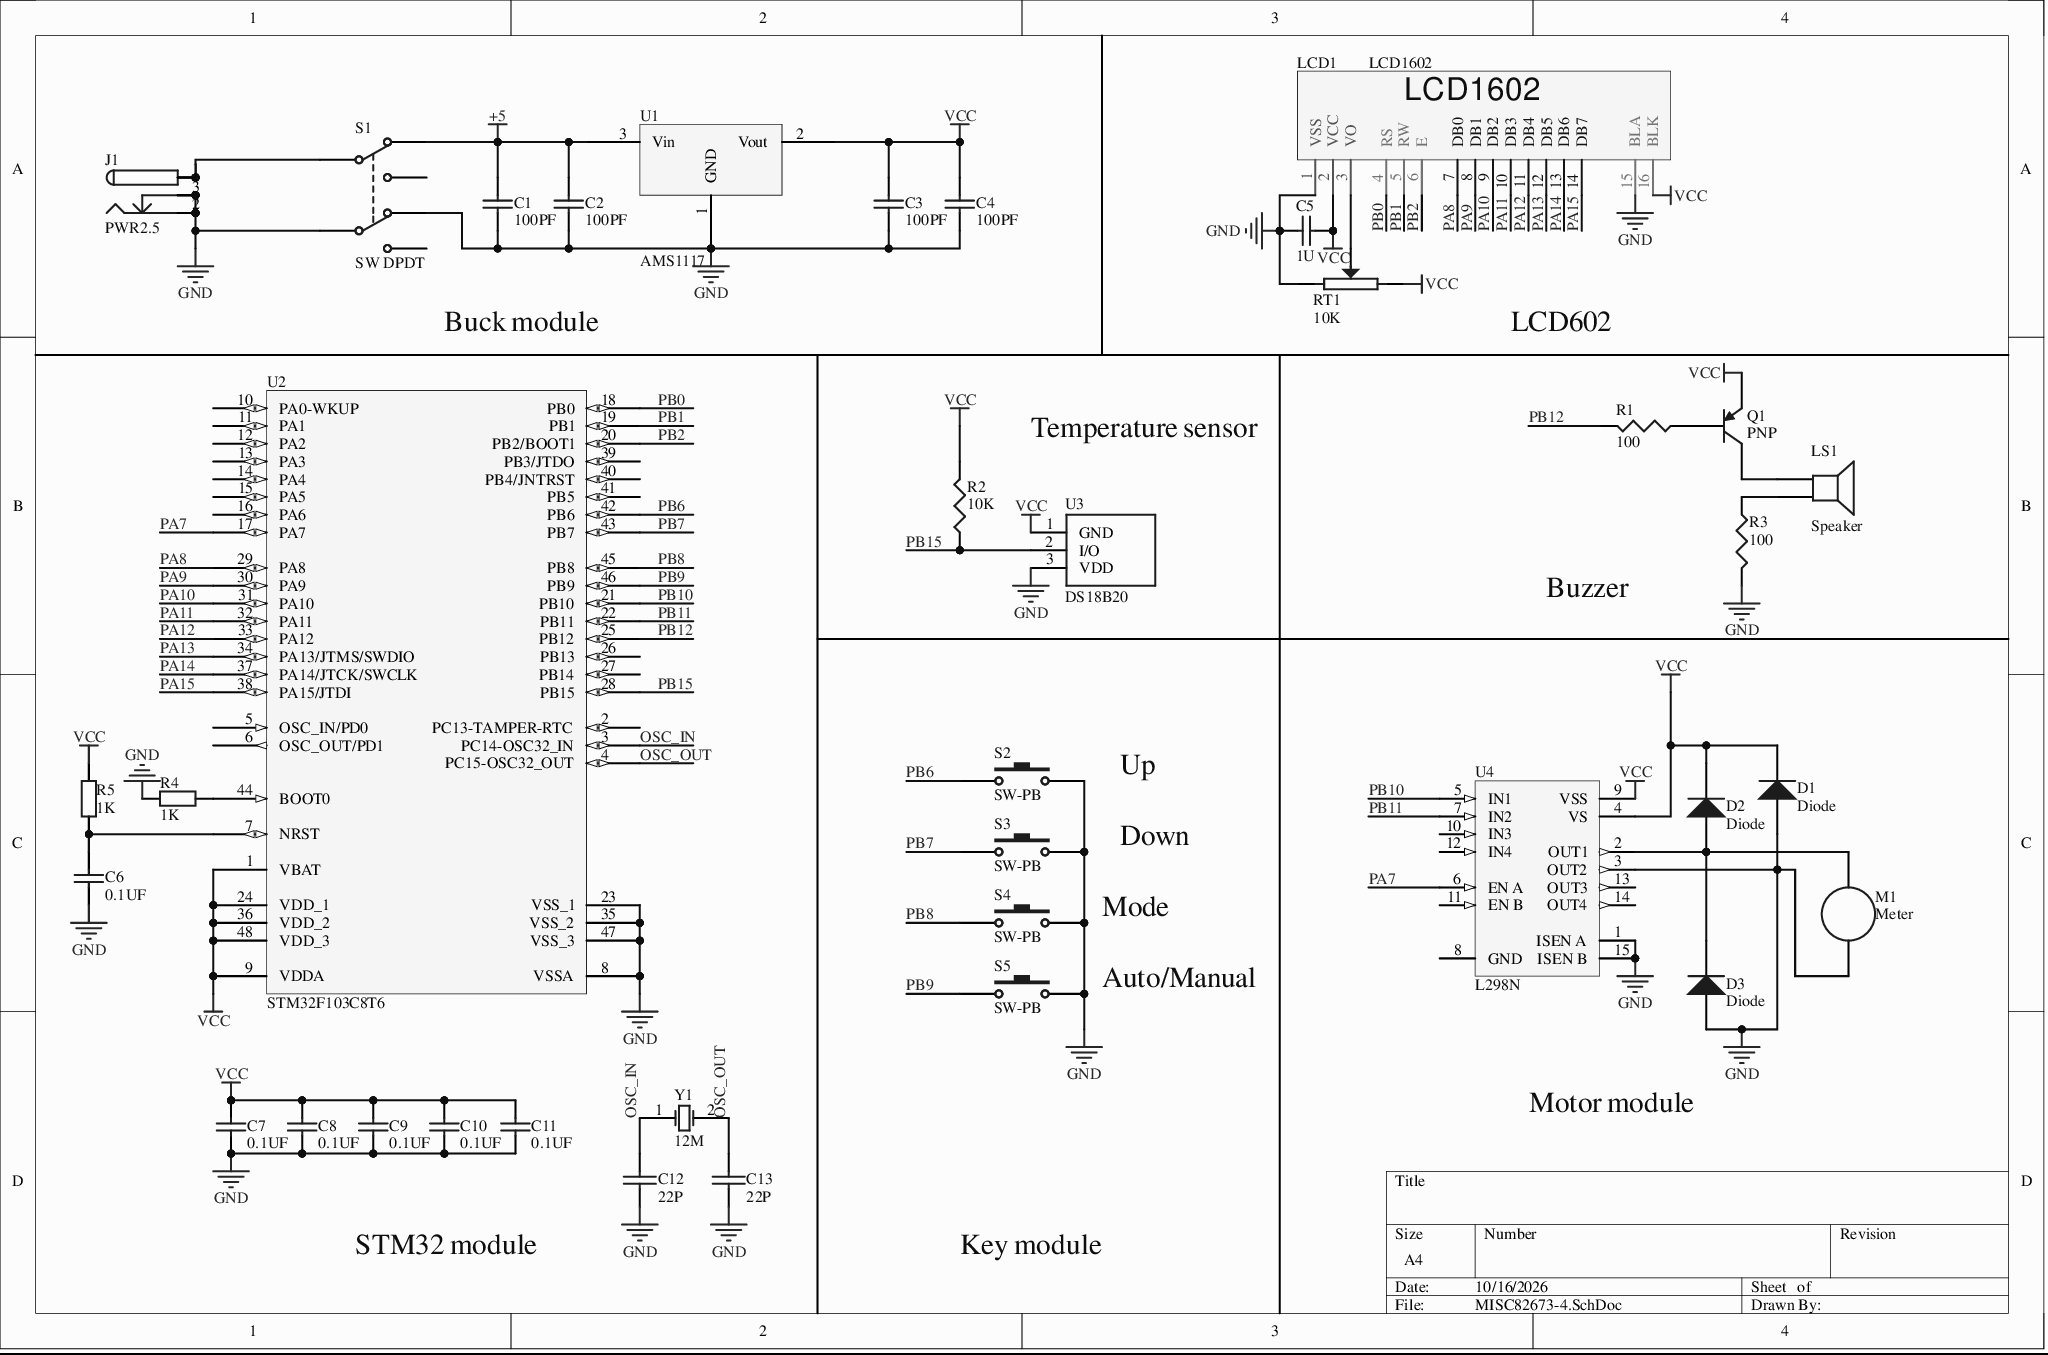
[diagram p0: MISC82673-4.SchDoc]
# Altium project MISC82673-7.PrjPcb
1 sheet, 37 parts. Net scope: global (net labels, ports and power ports of the same name join across sheets).
Board file: MISC82673.PcbDoc

## Sheet MISC82673-4.SchDoc
size A4

### Parts
C1  100PF  [C1206]
C2  100PF  [C1206]
C3  100PF  [C1206]
C4  100PF  [C1206]
C5  1U  [C1206]
C6  0.1UF  [C1206]
C7  0.1UF  [C1206]
C8  0.1UF  [C1206]
C9  0.1UF  [C1206]
C10  0.1UF  [C1206]
C11  0.1UF  [C1206]
C12  22P  [my0603]
C13  22P  [my0603]
D1  Diode  [SMC]
D2  Diode  [SMC]
D3  Diode  [SMC]
J1  PWR2.5  [KLD-0202]
LCD1  LCD1602  [LCD1602]
LS1  Speaker  [PIN2]
M1  Meter  [RAD-0.1]
Q1  PNP  [SOT-23B_N]
R1  100  [J1-0603]
R2  10K  [J1-0603]
R3  100  [J1-0603]
R4  value 1K  [my0603]  (hidden comment: Res2)
R5  value 1K  [my0603]  (hidden comment: Res2)
RT1  10K  [电位器]
S1  SW DPDT  [SOT23-6_N]
S2  SW-PB  [SW_PB2_A1]
S3  SW-PB  [SW_PB2_A1]
S4  SW-PB  [SW_PB2_A1]
S5  SW-PB  [SW_PB2_A1]
U1  AMS1117  [SOT223]
U2  STM32F103C8T6  [LQFP48 7X7]
U3  DS18B20  [HDR1X3]
U4  L298N  [Multiwatt15H]
Y1  12M  [XTAL_US]

### Nets
+5: C1.2 C2.2 S1.2(NC1) U1.3(Vin)
GND: C1.1 C2.1 C3.1 C4.1 C5.2 C6.1 C7.1 C8.1 C9.1 C10.1 C11.1 C12.2 C13.2 D1.1(A) D3.1(A) J1.2 J1.2A J1.2B J1.3 J1.3A J1.3B LCD1.1(VSS) LCD1.15(BLA) M1.1 R3.2 R4.2 RT1.1 S1.4(NC2) S1.5(COMMON2) S2.2 S3.2 S4.2 S5.2 U1.1(GND) U2.8(VSSA) U2.23(VSS_1) U2.35(VSS_2) U2.47(VSS_3) U3.3(VDD) U4.1(ISEN_A) U4.3(OUT2) U4.15(ISEN_B)
VCC: C3.2 C4.2 C5.1 C7.2 C8.2 C9.2 C10.2 C11.2 D1.2(K) D2.2(K) LCD1.2(VCC) LCD1.16(BLK) Q1.3(E) R2.2 R5.2 RT1.2 U1.2(Vout) U2.1(VBAT) U2.9(VDDA) U2.24(VDD_1) U2.36(VDD_2) U2.48(VDD_3) U3.1(GND) U4.4(VS) U4.9(VSS)
OSC_IN: C12.1 U2.3(PC14-OSC32_IN) Y1.1(OSC1)
OSC_OUT: C13.1 U2.4(PC15-OSC32_OUT) Y1.2(OSC2)
PA7: U2.17(PA7) U4.6(EN_A)
PA8: LCD1.7(DB0) U2.29(PA8)
PA9: LCD1.8(DB1) U2.30(PA9)
PA10: LCD1.9(DB2) U2.31(PA10)
PA11: LCD1.10(DB3) U2.32(PA11)
PA12: LCD1.11(DB4) U2.33(PA12)
PA13: LCD1.12(DB5) U2.34(PA13/JTMS/SWDIO)
PA14: LCD1.13(DB6) U2.37(PA14/JTCK/SWCLK)
PA15: LCD1.14(DB7) U2.38(PA15/JTDI)
PB0: LCD1.4(RS) U2.18(PB0)
PB1: LCD1.5(RW) U2.19(PB1)
PB2: LCD1.6(E) U2.20(PB2/BOOT1)
PB6: S2.1 U2.42(PB6)
PB7: S3.1 U2.43(PB7)
PB8: S4.1 U2.45(PB8)
PB9: S5.1 U2.46(PB9)
PB10: U2.21(PB10) U4.5(IN1)
PB11: U2.22(PB11) U4.7(IN2)
PB12: R1.2 U2.25(PB12)
PB15: R2.1 U2.28(PB15) U3.2(I/O)
NetC6_2: C6.2 R5.1 U2.7(NRST)
NetD2_1: D2.1(A) D3.2(K) M1.2 U4.2(OUT1)
NetJ1_1: J1.1 J1.1A J1.1B S1.1(COMMON1)
NetLCD1_3: LCD1.3(VO) RT1.3(W)
NetLS1_1: LS1.1 Q1.1(C)
NetLS1_2: LS1.2 R3.1
NetQ1_2: Q1.2(B) R1.1
NetR4_1: R4.1 U2.44(BOOT0)

Not connected (* = marked no-connect by the designer): S1 3(NO1) 6(NO2); U2 2(PC13-TAMPER-RTC) 5(OSC_IN/PD0) 6(OSC_OUT/PD1) 10(PA0-WKUP) 11(PA1) 12(PA2) 13(PA3) 14(PA4) 15(PA5) 16(PA6) 26(PB13) 27(PB14) 39(PB3/JTDO) 40(PB4/JNTRST) 41(PB5); U4 8(GND) 10(IN3) 11(EN_B) 12(IN4) 13(OUT3) 14(OUT4)

### Notes on the sheet
- Buck module
- LCD602
- Temperature sensor
- Buzzer
- Up
- Down
- Mode
- Auto/Manual
- Motor module
- STM32 module
- Key module

### Library data of the parts
C1-C4 = Cap Semi: Capacitor (Semiconductor SIM Model); Published: 8-Jun-2000; LatestRevisionDate: 29-May-2009; LatestRevisionNote: IPC-7351 Footprint Added.; PackageReference: C1206; PackageDescription: Chip Capacitor; Value: 100pF; Publisher: Altium Limited
C5-C11 = Cap Semi: Capacitor (Semiconductor SIM Model); Value: 100pF; Published: 8-Jun-2000; LatestRevisionDate: 29-May-2009; LatestRevisionNote: IPC-7351 Footprint Added.; PackageReference: C1206; PackageDescription: Chip Capacitor; Publisher: Altium Limited
C12 C13 = CAP: Capacitor
D1-D3 = Diode: Default Diode; Published: 8-Jun-2000; LatestRevisionDate: 17-Jul-2002; LatestRevisionNote: Re-released for DXP Platform.; PackageVersion: Sep-1996; PackageReference: SMC; PackageDescription: DO-214-AB/SMC; 2 C-Bend Leads; Body 7.9 x 5.9 mm, inc. leads (LxW); Code_JEDEC: DO-214-AB; Publisher: Altium Limited
J1 = PWR2.5: Low Voltage Power Supply Connector; Published: 17-Dec-2003; DatasheetDocument: 09-May-2002; ComponentLink1Description: Manufacturer Link; Publisher: Altium Limited
LS1 = Speaker: Loudspeaker; Published: 24-Mar-1999; LatestRevisionDate: 17-Jul-2002; LatestRevisionNote: Re-released for DXP Platform.; PackageReference: PIN2; Publisher: Altium Limited
M1 = Meter: Indicating Instrument; Note: Place a "letter" into the symbol to show the function of the meter or instrument; Published: 24-Mar-1999; LatestRevisionDate: 17-Jul-2002; LatestRevisionNote: Re-released for DXP Platform.; PackageReference: RAD-0.1; PackageDescription: Radial Cap, Thru-Hole; 2 Leads; 0.1 in Pin Spacing; Publisher: Altium Limited
Q1 = PNP: PNP Bipolar Transistor; Published: 8-Jun-2000; LatestRevisionDate: 29-May-2009; LatestRevisionNote: IPC-7351 Footprint Added.; PackageVersion: Aug-1999; PackageReference: SOT-23B; PackageDescription: 3-Pin SOT-23 Package 0.95 mm Pitch, 2.4 mm Lead Span; Publisher: Altium Limited
R1-R3 = Res3: Resistor; Value: 1K; Published: 8-Jun-2000; LatestRevisionDate: 29-May-2009; LatestRevisionNote: IPC-7351 Footprint Added.; PackageReference: J1-0603; PackageDescription: Chip Resistor; Publisher: Altium Limited
R4 R5 = Res2: Resistor; Published: 8-Jun-2000; LatestRevisionDate: 17-Jul-2002; LatestRevisionNote: Re-released for DXP Platform.; PackageReference: AXIAL-0.4; PackageDescription: Axial Device, Thru-Hole; 2 Leads; 0.4 in Pin Spacing; Publisher: Altium Limited
RT1 = 电位器
S1 = SW DPDT: Switch; Published: 24-Mar-1999; LatestRevisionDate: 29-May-2009; LatestRevisionNote: IPC-7351 Footprint Added.; PackageVersion: Mar-2001; PackageReference: SOT23-6; PackageDescription: 6-Pin SOT-23 Package 0.95 mm Pitch, 2.7 mm Lead Span; Code_JEITA: SC-74; Code_IPC: SOT26A-6; Publisher: Altium Limited
S2-S5 = SW-PB: Switch; Published: 24-Mar-1999; LatestRevisionDate: 17-Jul-2002; LatestRevisionNote: Re-released for DXP Platform.; Publisher: Altium Limited
U1 = AMS1117: Three-terminal voltage regulator
U4 = L298N: Dual Full Bridge Driver; Revision 1: 24-Aug-2001: Footprint Added.; Revision 2: 17-Jul-2002: Re-released for DXP Platform.; Package Information: Latest Revision: Apr-1998; Published: 8-Jun-2000; Datasheet: Latest Revision: Jul-1999; Package Reference: Multiwatt15H; Publisher: Altium Limited
Y1 = XTAL: Crystal Oscillator; Published: 8-Jun-2000; LatestRevisionDate: 17-Jul-2002; LatestRevisionNote: Re-released for DXP Platform.; Publisher: Altium Limited